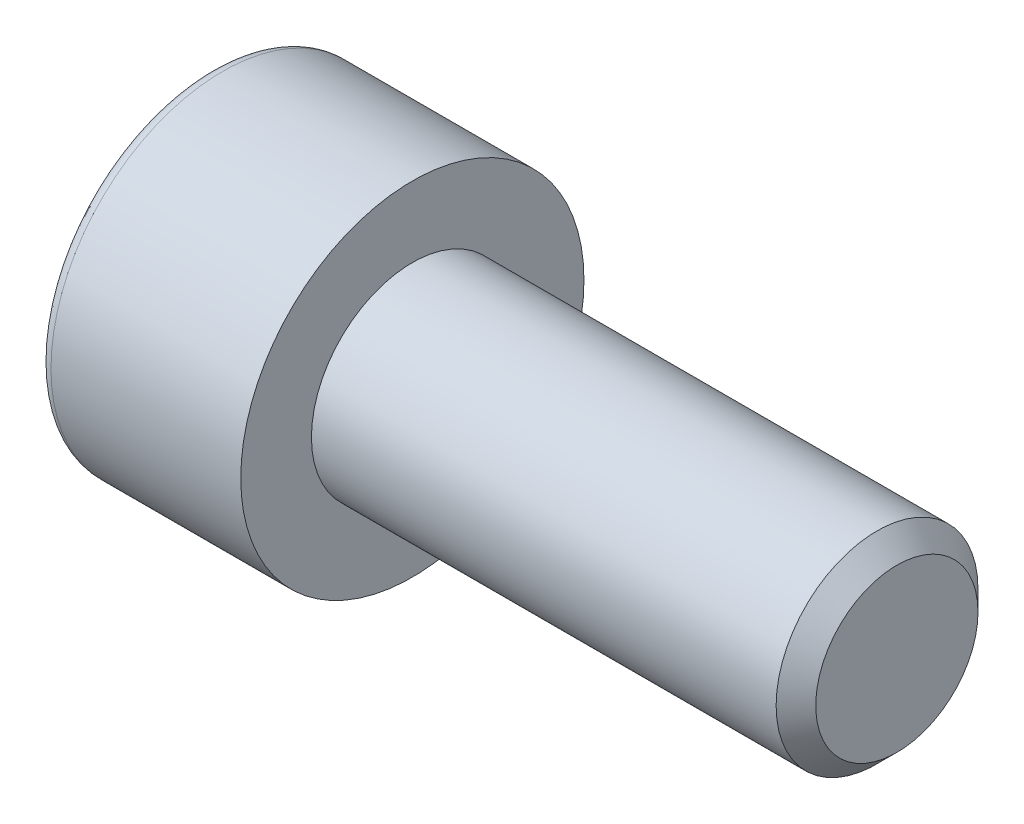
SolidWorks part; units mm, degrees
ref_plane "前视基准面" through (0, 0, 0) normal (0, 0, 1) x (1, 0, 0)
ref_plane "上视基准面" through (0, 0, 0) normal (0, 1, 0) x (1, 0, 0)
ref_plane "右视基准面" through (0, 0, 0) normal (1, 0, 0) x (0, 0, -1)
sketch "草图1" plane through (0, 0, 0) normal (0, 0, 1) x (1, 0, 0)
  line L0 (17, 0) -> (17, -2.0095)
  line L1 (17, -2.0095) -> (16.5095, -2.5)
  line L2 (16.5095, -2.5) -> (5, -2.5)
  line L3 (5, -2.5) -> (5, -4.25)
  line L4 (5, -4.25) -> (0.3, -4.25)
  line L5 (0, -3.95) -> (0, 0)
  line L6 (0, 0) -> (17, 0)
  line L7 (0, 0) -> (17, 0) construction
  arc A0 (0.3, -4.25) -> (0, -3.95) centre (0.3, -3.95) cw
revolve "旋转1" add sketch "草图1" angle 360 about L7
cosmetic thread "装饰螺纹线1"
sketch "草图2" plane through (0, 0, 0) normal (1, 0, 0) x (0, 0, -1)
  line L0 (-1.7, -0.9815) -> (0, -1.963)
  line L1 (0, -1.963) -> (1.7, -0.9815)
  line L2 (1.7, -0.9815) -> (1.7, 0.9815)
  line L3 (1.7, 0.9815) -> (0, 1.963)
  line L4 (0, 1.963) -> (-1.7, 0.9815)
  line L5 (-1.7, 0.9815) -> (-1.7, -0.9815)
extrude "切除-拉伸1" cut sketch "草图2" along normal blind 2.5
